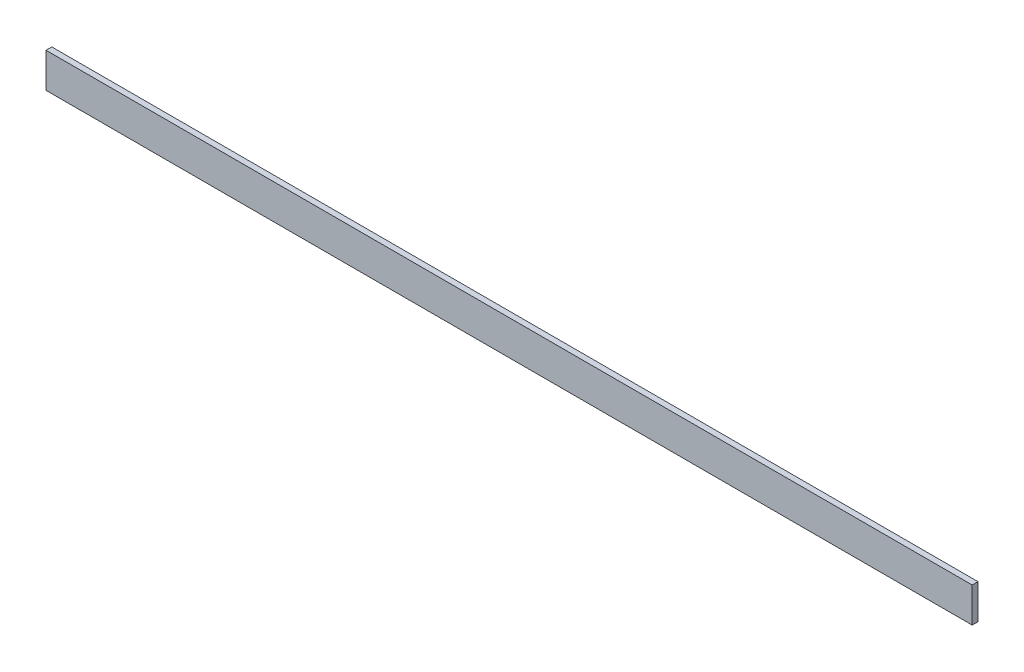
from build123d import *

# Parameters (mm, degrees)
SKETCH1_W           = 800
SKETCH1_H           = 30
BOSS_EXTRUDE1_DEPTH = 5


with BuildPart() as part:
    # Sketch1 → Boss-Extrude1 (new body)
    with BuildSketch(Plane.XY):
        Rectangle(SKETCH1_W, SKETCH1_H)
    extrude(amount=BOSS_EXTRUDE1_DEPTH)


solid = part.part
